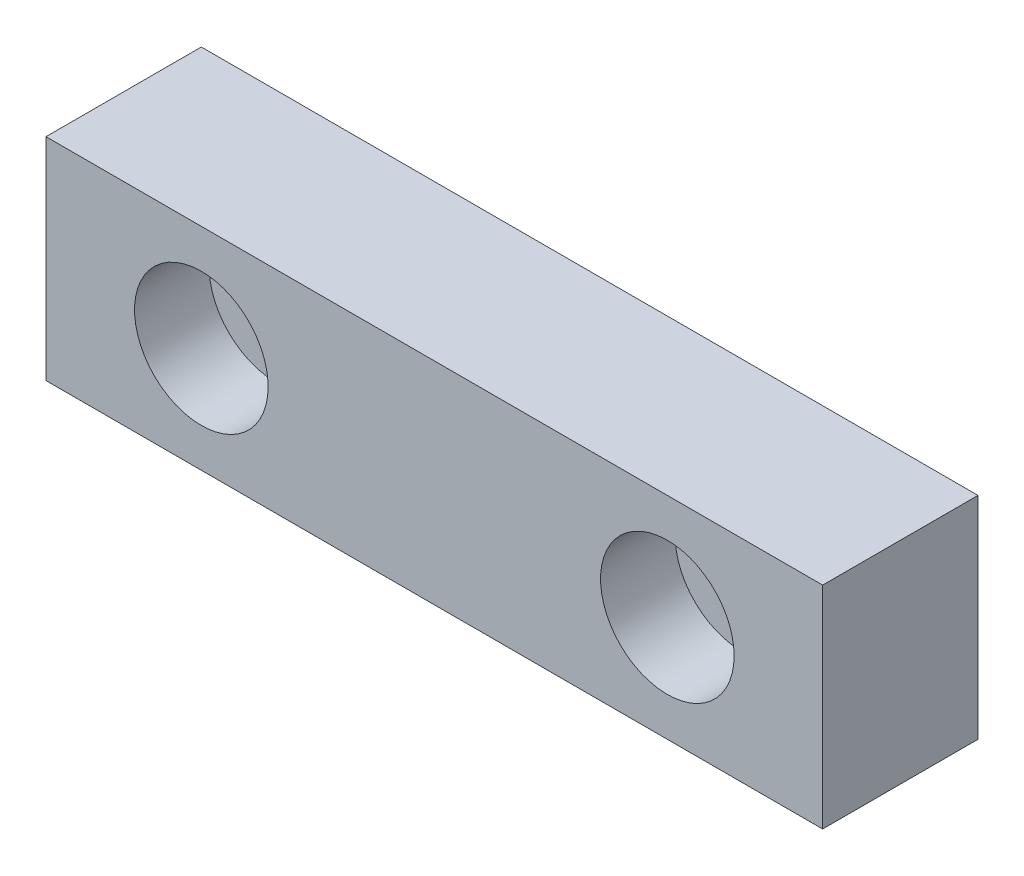
from build123d import *

# Parameters (mm, degrees)
SKETCH_1_W          = 25
SKETCH_1_H          = 6.8
EXTRUDE_1_DEPTH     = 5
CUT_EXTRUDE_1_REACH = 19.791
SKETCH_2_R          = 1.2
SKETCH_3_R          = 2.15
CUT_EXTRUDE_2_DEPTH = 2.4


with BuildPart() as part:
    # 草图1 → 凸台-拉伸1 (new body)
    with BuildSketch(Plane.XY):
        with Locations((4.154545455, -0.360606061)):
            Rectangle(SKETCH_1_W, SKETCH_1_H)
    extrude(amount=EXTRUDE_1_DEPTH)

    # 草图2 → 切除-拉伸1 (cut, up to next)
    with BuildSketch(Plane.XY.offset(5), mode=Mode.PRIVATE) as cut_extrude_1_sk1:
        with Locations((-3.345454545, -0.360606061)):
            Circle(SKETCH_2_R)
    cut_extrude_1_tool1 = extrude(cut_extrude_1_sk1.sketch, amount=-CUT_EXTRUDE_1_REACH, mode=Mode.PRIVATE) & part.part
    # 草图2 → 切除-拉伸1 (cut, up to next)
    with BuildSketch(Plane.XY.offset(5), mode=Mode.PRIVATE) as cut_extrude_1_sk2:
        with Locations((11.654545455, -0.360606061)):
            Circle(SKETCH_2_R)
    cut_extrude_1_tool2 = extrude(cut_extrude_1_sk2.sketch, amount=-CUT_EXTRUDE_1_REACH, mode=Mode.PRIVATE) & part.part
    add(cut_extrude_1_tool1.solids().sort_by_distance((-3.345455, -0.360606, 5))[0], mode=Mode.SUBTRACT)
    add(cut_extrude_1_tool2.solids().sort_by_distance((11.654545, -0.360606, 5))[0], mode=Mode.SUBTRACT)

    # 草图3 → 切除-拉伸2 (cut)
    with BuildSketch(Plane.XY.offset(5)):
        with Locations((-3.345454545, -0.360606061)):
            Circle(SKETCH_3_R)
        with Locations((11.654545455, -0.360606061)):
            Circle(SKETCH_3_R)
    extrude(amount=-CUT_EXTRUDE_2_DEPTH, mode=Mode.SUBTRACT)


solid = part.part
